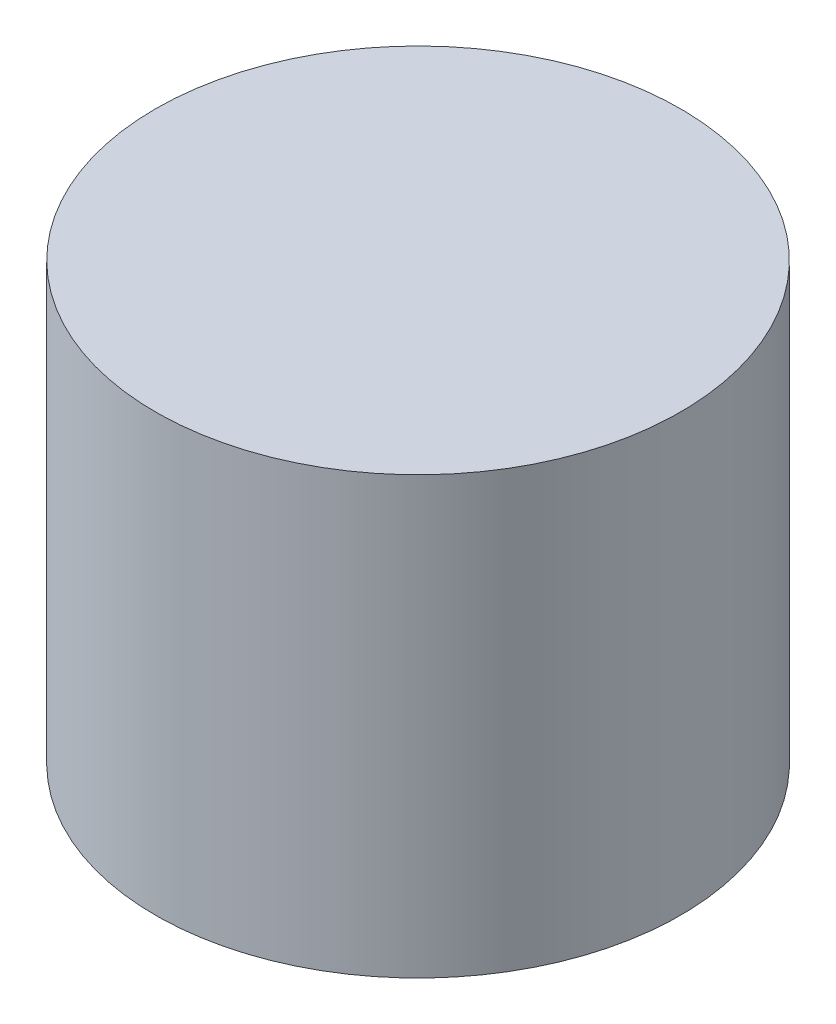
from build123d import *


with BuildPart() as part:
    # Sketch2 → Revolve1 (revolve)
    with BuildSketch(Plane.XY):
        Polygon((-8.5, 14), (-8.5, -0.10996164), (-8, -0.10996164), (-5.101647841, 3.344159959), (-5.101647841, 4.665808374), (-6.5, 4.665808374), (-6.5, 13), (0, 13), (0, 14), align=None)
    revolve(axis=Axis((0, 14, 0), (0, -1, 0)))


solid = part.part
